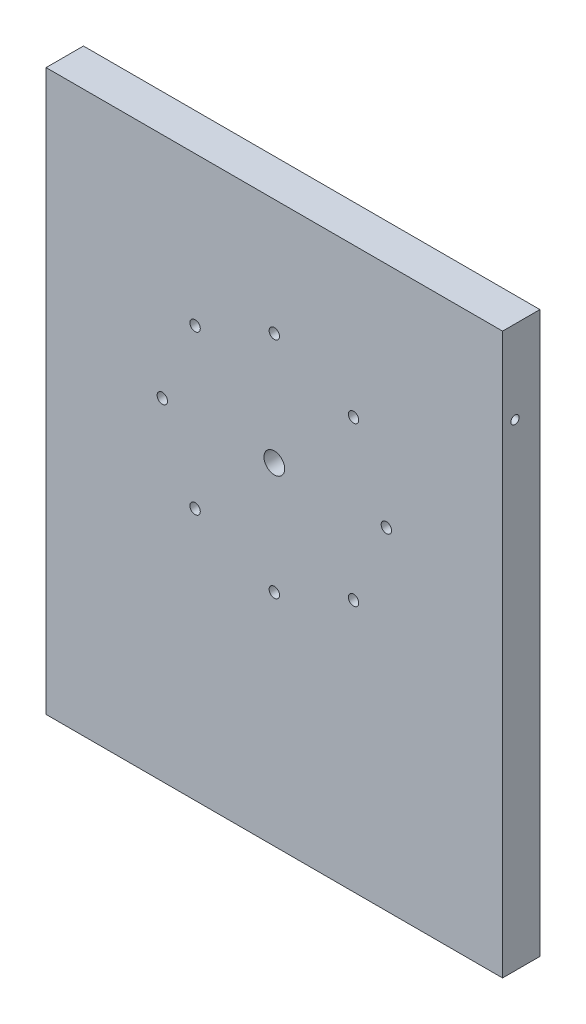
SolidWorks part; units mm, degrees
material "6061-T6 (SS)"
ref_plane "前视基准面" through (0, 0, 0) normal (0, 0, 1) x (1, 0, 0)
ref_plane "上视基准面" through (0, 0, 0) normal (0, 1, 0) x (1, 0, 0)
ref_plane "右视基准面" through (0, 0, 0) normal (1, 0, 0) x (0, 0, -1)
other "Configuration Table"
sketch "草图1" plane through (0, 0, 0) normal (0, 0, 1) x (1, 0, 0)
  line L1 (-110, -140) -> (110, -140)
  line L2 (-110, -140) -> (-110, 140)
  line L3 (-110, 140) -> (110, 140)
  line L4 (110, -140) -> (110, 140)
  line L5 (-110, -140) -> (110, 140) construction
  line L6 (-110, 140) -> (110, -140) construction
  point P0 (0, 0)
  dimension "D1" = 220
  dimension "D2" = 280
extrude "凸台-拉伸1" add sketch "草图1" along normal blind 18
sketch "草图2" plane through (0, 0, 0) normal (0, 0, 1) x (1, 0, 0)
  line L1 (110, -140) -> (110, 140) construction
  line L2 (110, -80) -> (-110, -80)
  line L3 (-110, 140) -> (-110, -140) construction
  line L4 (-110, -80) -> (-110, -140)
  line L5 (-110, -140) -> (110, -140)
  line L6 (110, -140) -> (110, -80)
extrude "切除-拉伸1" cut sketch "草图2" along normal through all
sketch "草图4" plane through (0, 0, 0) normal (0, 0, 1) x (1, 0, 0)
  circle A0 centre (0, 30) radius 5
  dimension "D1" = 10
extrude "切除-拉伸3" cut sketch "草图4" along normal through all
sketch "草图5" plane through (0, 0, 0) normal (0, 0, -1) x (-1, 0, 0)
  circle A2 centre (-38.1838, 68.1838) radius 2.5
  circle A3 centre (0, 84) radius 2.5
  circle A4 centre (-54, 30) radius 2.5
  circle A5 centre (-38.1838, -8.1838) radius 2.5
  circle A6 centre (0, -24) radius 2.5
  circle A7 centre (38.1838, -8.1838) radius 2.5
  circle A8 centre (54, 30) radius 2.5
  circle A9 centre (38.1838, 68.1838) radius 2.5
  point P21 (0, 30)
  dimension "D2" = 8
  dimension "D3" = 5
extrude "切除-拉伸4" cut sketch "草图5" against normal through all
sketch "草图13" plane through (-110, 0, 0) normal (-1, 0, 0) x (0, 0, 1)
  line L1 (0, -80) -> (18, -80)
  line L2 (0, -80) -> (0, -130)
  line L3 (0, -130) -> (18, -130)
  line L4 (18, -80) -> (18, -130)
  dimension "D1" = 50
extrude "凸台-拉伸2" add sketch "草图13" against normal through all
sketch "草图15" plane through (110, 0, 0) normal (1, 0, 0) x (0, 0, -1)
  circle A0 centre (-12, 100) radius 2
  dimension "D3" = 4
extrude "切除-拉伸5" cut sketch "草图15" against normal through all
